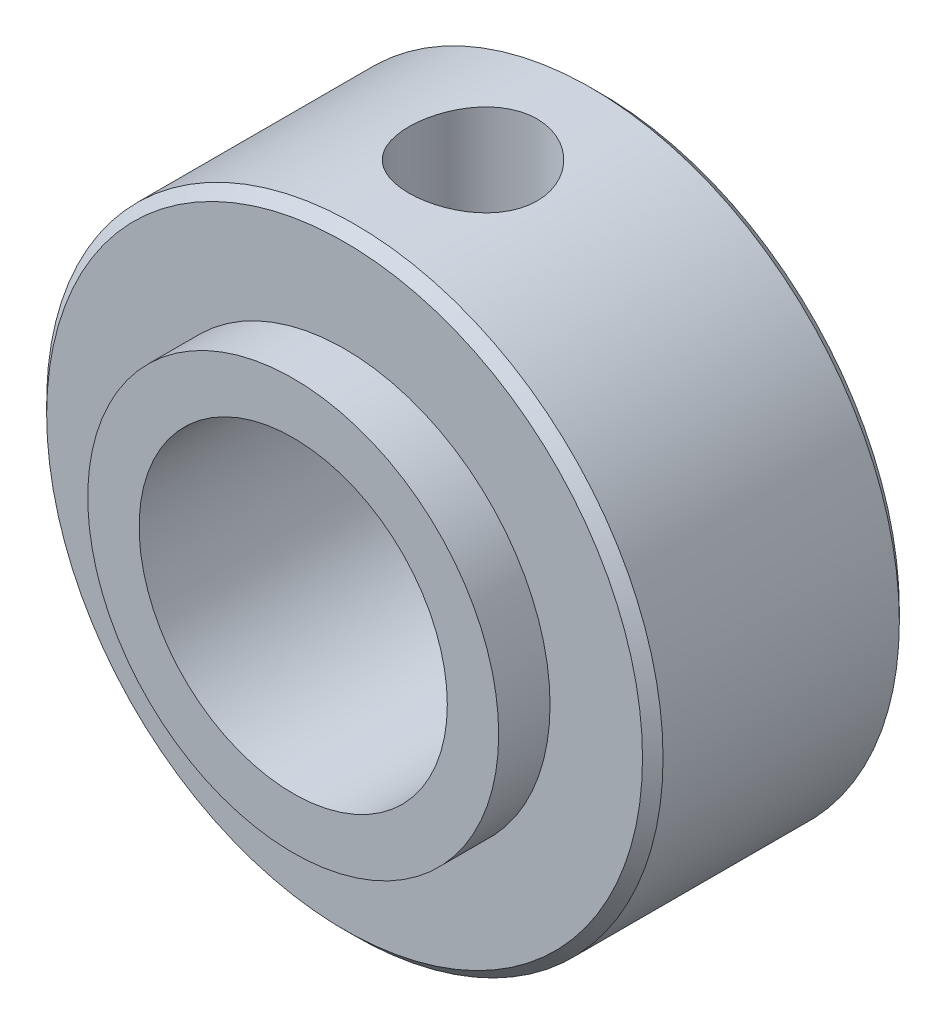
SolidWorks part; units mm, degrees
ref_plane "Front Plane" through (0, 0, 0) normal (0, 0, 1) x (1, 0, 0)
ref_plane "Top Plane" through (0, 0, 0) normal (0, 1, 0) x (1, 0, 0)
ref_plane "Right Plane" through (0, 0, 0) normal (1, 0, 0) x (0, 0, -1)
sketch "Sketch1" plane through (0, 0, 0) normal (0, 0, 1) x (1, 0, 0)
  circle A0 centre (0, 0) radius 6
  dimension "D1" = 12
extrude "Boss-Extrude1" add sketch "Sketch1" along normal blind 5
sketch "Sketch2" plane through (0, 0, 5) normal (0, 0, 1) x (1, 0, 0)
  circle A0 centre (0, 0) radius 4
  dimension "D1" = 8
extrude "Boss-Extrude2" add sketch "Sketch2" along normal blind 1
sketch "Sketch3" plane through (0, 0, 6) normal (0, 0, 1) x (1, 0, 0)
  circle A0 centre (0, 0) radius 3
  dimension "D1" = 6
extrude "Cut-Extrude1" cut sketch "Sketch3" against normal through all
chamfer "Chamfer1" distance 0.2 angle 45 2 edges at (6, 0, 0) (6, 0, 5)
hole_wizard "M3 Tapped Hole1" positions "Sketch5" profile "Sketch4" tap size "M3" standard "GB"
sketch "Sketch5" plane through (0, 0, 0) normal (0, 1, 0) x (1, 0, 0)
  point P0 (0, -2.5)
  dimension "D1" = 2.5
sketch "Sketch4" plane through (0, 0, 2.5) normal (1, 0, 0) x (0, 0, -1)
  line L0 (0, 0) -> (0, 8.2511)
  line L1 (0, 8.2511) -> (1.25, 7.5)
  line L2 (1.25, 7.5) -> (1.25, 0)
  line L5 (1.25, 0) -> (0, 0)
  line L10 (0, 8.2511) -> (-1.25, 7.5) construction
  line L11 (0, -6.35) -> (0, 107.95) construction
  dimension "螺纹孔钻头直径" = 2.5
  dimension "螺纹孔钻头深度" = 7.5
  dimension "导头角度" = 118
cosmetic thread "Cosmetic Thread1" parameters "D1"=6, "D2"=3
